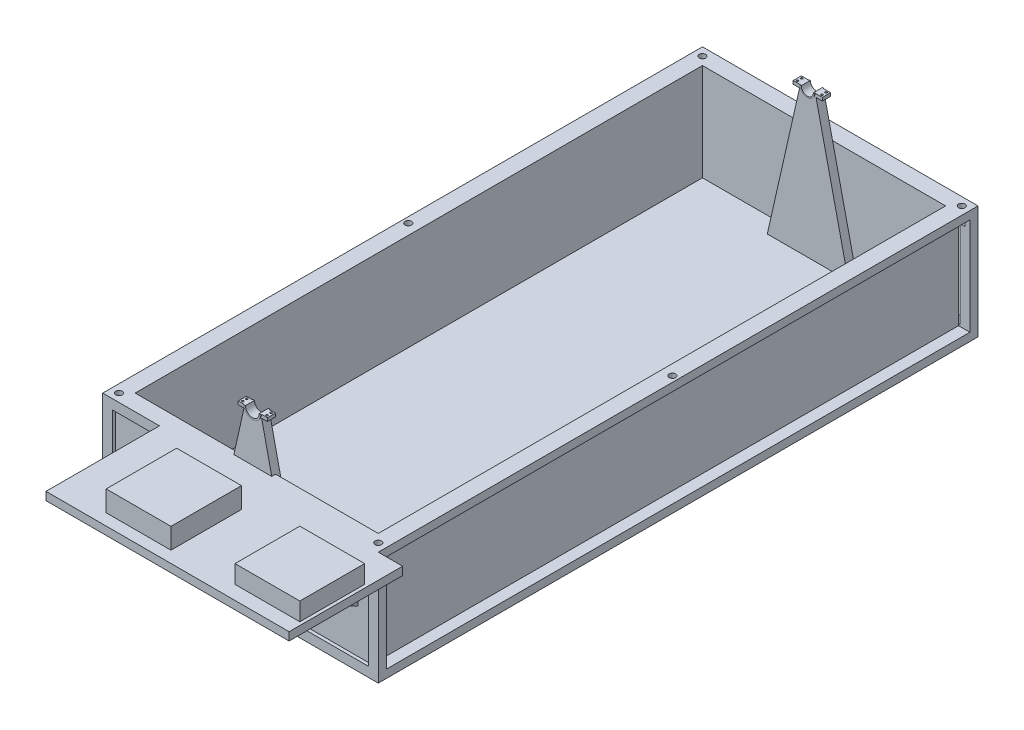
from build123d import *

# Parameters (mm, degrees)
SKETCH_1_R             = 50
SKETCH_1_R_2           = 42.55
EXTRUDE_1_DEPTH        = 50
SKETCH_3_R             = 45
SKETCH_3_R_2           = 37.55
EXTRUDE_2_DEPTH        = 50
EXTRUDE_START          = -50
EXTRUDE_3_DEPTH        = 50
SKETCH_8_R             = 37.55
EXTRUDE_4_DEPTH        = 50
SKETCH_4_W             = 700
SKETCH_4_H             = 3700
EXTRUDE_5_DEPTH        = 100
SKETCH_12_W            = 500
SKETCH_12_H            = 1000
EXTRUDE_6_DEPTH        = 100
SKETCH_16_W            = 500
SKETCH_16_H            = 2700
EXTRUDE_8_DEPTH        = 100
SKETCH_17_W            = 100
SKETCH_17_H            = 100
EXTRUDE_9_DEPTH        = 600
SKETCH_18_W            = 100
SKETCH_18_H            = 100
EXTRUDE_10_DEPTH       = 600
SKETCH_19_W            = 100
SKETCH_19_H            = 100
EXTRUDE_11_DEPTH       = 3500
SKETCH_20_R            = 25
CUT_EXTRUDE_5_DEPTH    = 20
SKETCH_21_R            = 52.5
SKETCH_21_R_2          = 42.55
EXTRUDE_12_DEPTH       = 50
CUT_EXTRUDE_START      = -356
CUT_EXTRUDE_6_DEPTH    = 356
SKETCH_23_W            = 47.45
SKETCH_23_H            = 50
EXTRUDE_13_DEPTH       = 20
CUT_EXTRUDE_8_DEPTH    = 611
SKETCH_26_W            = 52.45
SKETCH_26_H            = 50
EXTRUDE_14_DEPTH       = 20
SKETCH_27_R            = 6
CUT_EXTRUDE_9_DEPTH    = 20
SKETCH_28_R            = 6
CUT_EXTRUDE_10_DEPTH   = 20
EXTRUDE_START_2        = -53
EXTRUDE_15_DEPTH       = 53
EXTRUDE_START_3        = 3
EXTRUDE_16_DEPTH       = 3
EXTRUDE_17_DEPTH       = 3
EXTRUDE_18_DEPTH       = 53
SKETCH_31_W            = 3500
SKETCH_31_H            = 500
EXTRUDE_19_DEPTH       = 100
SKETCH_33_W            = 500
SKETCH_33_H            = 3700
EXTRUDE_20_DEPTH       = 100
EXTRUDE_21_DEPTH       = 100
SKETCH_35_W            = 1500
SKETCH_35_H            = 600
EXTRUDE_22_DEPTH       = 100
SKETCH_36_W            = 1500
SKETCH_36_H            = 600
EXTRUDE_23_DEPTH       = 100
SKETCH_37_W            = 3600
SKETCH_37_H            = 600
CUT_EXTRUDE_11_DEPTH   = 70
SKETCH_38_W            = 1580
SKETCH_38_H            = 580
CUT_EXTRUDE_15_DEPTH   = 50
SKETCH_39_W            = 3600
SKETCH_39_H            = 600
CUT_EXTRUDE_16_DEPTH   = 70
SKETCH_40_W            = 1580
SKETCH_40_H            = 580
CUT_EXTRUDE_17_DEPTH   = 20
SKETCH_43_R            = 20
CUT_EXTRUDE_20_DEPTH   = 100
EXTRUDE_24_DEPTH       = 50
EXTRUDE_25_DEPTH       = 25
PATTERN_LINEAR_1_COUNT = 4
PATTERN_LINEAR_1_PITCH = 100
PATTERN_LINEAR_2_COUNT = 8
PATTERN_LINEAR_2_PITCH = 100
SKETCH_46_W            = 400
SKETCH_46_H            = 435
EXTRUDE_26_DEPTH       = 127.5
SKETCH_47_W            = 400
SKETCH_47_H            = 400
EXTRUDE_28_DEPTH       = 111


with BuildPart() as part:
    # 草图1 → 凸台-拉伸1 (new body)
    with BuildSketch(Plane.XY):
        Circle(SKETCH_1_R)
        Circle(SKETCH_1_R_2, mode=Mode.SUBTRACT)
    extrude(amount=EXTRUDE_1_DEPTH)

    # 草图7 → 凸台-拉伸3 (add)
    with BuildSketch(Plane.XY.offset(50).offset(EXTRUDE_START)):
        with BuildLine():
            ThreePointArc((50, 0), (0, -50), (-50, 0))
            Line((-50, 0), (-250, -900))
            Line((-250, -900), (250, -900))
            Line((250, -900), (50, 0))
        make_face()
    extrude(amount=EXTRUDE_3_DEPTH)



with BuildPart() as body_2:
    # 草图3 → 凸台-拉伸2 (new body)
    with BuildSketch(Plane(origin=(0, 0, -3374), x_dir=(-1, 0, 0), z_dir=(0, 0, -1))):
        Circle(SKETCH_3_R)
        Circle(SKETCH_3_R_2, mode=Mode.SUBTRACT)
    extrude(amount=EXTRUDE_2_DEPTH)

    # 草图8 → 凸台-拉伸4 (add)
    with BuildSketch(Plane(origin=(0, 0, -3424), x_dir=(-1, 0, 0), z_dir=(0, 0, -1))):
        with BuildLine():
            Line((-43.888190419, 9.941164005), (-250, -900))
            Line((-250, -900), (250, -900))
            Line((250, -900), (43.888190419, 9.941164005))
            ThreePointArc((43.888190419, 9.941164005), (0, 45), (-43.888190419, 9.941164005))
        make_face()
        Circle(SKETCH_8_R, mode=Mode.SUBTRACT)
    extrude(amount=-EXTRUDE_4_DEPTH)


with BuildPart() as part_1:
    add(part.part)

    add(body_2.part)  # 凸台-拉伸5 merges body 2
    # 草图4 → 凸台-拉伸5 (add)
    with BuildSketch(Plane(origin=(0, -900, 0), x_dir=(1, 0, 0), z_dir=(0, 1, 0))):
        with Locations((0, 1724)):
            Rectangle(SKETCH_4_W, SKETCH_4_H)
    extrude(amount=-EXTRUDE_5_DEPTH)

    # 草图12 → 凸台-拉伸6 (add)
    with BuildSketch(Plane(origin=(0, -900, 0), x_dir=(1, 0, 0), z_dir=(0, 1, 0))):
        with Locations((600, 374)):
            Rectangle(SKETCH_12_W, SKETCH_12_H)
    extrude(amount=-EXTRUDE_6_DEPTH)

    # 草图16 → 凸台-拉伸8 (add)
    with BuildSketch(Plane(origin=(0, -900, 0), x_dir=(1, 0, 0), z_dir=(0, 1, 0))):
        with Locations((600, 2224)):
            Rectangle(SKETCH_16_W, SKETCH_16_H)
    extrude(amount=-EXTRUDE_8_DEPTH)

    # 草图17 → 凸台-拉伸9 (add)
    with BuildSketch(Plane(origin=(0, -900, 0), x_dir=(1, 0, 0), z_dir=(0, 1, 0))):
        with Locations((800, 3524)):
            Rectangle(SKETCH_17_W, SKETCH_17_H)
    extrude(amount=EXTRUDE_9_DEPTH)

    # 草图18 → 凸台-拉伸10 (add)
    with BuildSketch(Plane(origin=(0, -900, 0), x_dir=(1, 0, 0), z_dir=(0, 1, 0))):
        with Locations((800, -76)):
            Rectangle(SKETCH_18_W, SKETCH_18_H)
    extrude(amount=EXTRUDE_10_DEPTH)

    # 草图19 → 凸台-拉伸11 (add)
    with BuildSketch(Plane.XY.offset(-3474)):
        with Locations((800, -350)):
            Rectangle(SKETCH_19_W, SKETCH_19_H)
    extrude(amount=EXTRUDE_11_DEPTH)

    # 草图20 → 切除-拉伸5 (cut)
    with BuildSketch(Plane.ZY.offset(-750)):
        with Locations((-3424, -350)):
            Circle(SKETCH_20_R)
    extrude(amount=-CUT_EXTRUDE_5_DEPTH, mode=Mode.SUBTRACT)

    # 草图21 → 凸台-拉伸12 (add)
    with BuildSketch(Plane.XY.offset(50).offset(EXTRUDE_START)):
        Circle(SKETCH_21_R)
        Circle(SKETCH_21_R_2, mode=Mode.SUBTRACT)
    extrude(amount=EXTRUDE_12_DEPTH)

    # 草图22 → 切除-拉伸6 (cut)
    with BuildSketch(Plane.XY.offset(50).offset(CUT_EXTRUDE_START)):
        with BuildLine():
            Line((-52.5, 0), (52.5, 0))
            ThreePointArc((52.5, 0), (0, 52.5), (-52.5, 0))
        make_face()
    extrude(amount=CUT_EXTRUDE_6_DEPTH, mode=Mode.SUBTRACT)

    # 草图23 → 凸台-拉伸13 (add)
    with BuildSketch(Plane(origin=(0, 0, 0), x_dir=(1, 0, 0), z_dir=(0, 1, 0))):
        with Locations((-66.275, -25)):
            Rectangle(SKETCH_23_W, SKETCH_23_H)
        with Locations((66.275, -25)):
            Rectangle(SKETCH_23_W, SKETCH_23_H)
    extrude(amount=-EXTRUDE_13_DEPTH)

    # 草图24 → 切除-拉伸8 (cut)
    with BuildSketch(Plane(origin=(0, 0, -3424), x_dir=(-1, 0, 0), z_dir=(0, 0, -1))):
        with BuildLine():
            Line((-55, 0), (55, 0))
            ThreePointArc((55, 0), (0, 55), (-55, 0))
        make_face()
    extrude(amount=-CUT_EXTRUDE_8_DEPTH, mode=Mode.SUBTRACT)

    # 草图26 → 凸台-拉伸14 (add)
    with BuildSketch(Plane(origin=(0, 0, 0), x_dir=(1, 0, 0), z_dir=(0, 1, 0))):
        with Locations((-63.775, 3399)):
            Rectangle(SKETCH_26_W, SKETCH_26_H)
        with Locations((63.775, 3399)):
            Rectangle(SKETCH_26_W, SKETCH_26_H)
    extrude(amount=-EXTRUDE_14_DEPTH)

    # 草图27 → 切除-拉伸9 (cut)
    with BuildSketch(Plane(origin=(0, 0, 0), x_dir=(1, 0, 0), z_dir=(0, 1, 0))):
        with Locations(Location((-75, -12.5, 0), (0, 0, 270))):
            Circle(SKETCH_27_R)
        with Locations(Location((-75, -37.5, 0), (0, 0, 270))):
            Circle(SKETCH_27_R)
        with Locations(Location((75, -37.5, 0), (0, 0, 90))):
            Circle(SKETCH_27_R)
        with Locations(Location((75, -12.5, 0), (0, 0, 90))):
            Circle(SKETCH_27_R)
    extrude(amount=-CUT_EXTRUDE_9_DEPTH, mode=Mode.SUBTRACT)

    # 草图28 → 切除-拉伸10 (cut)
    with BuildSketch(Plane(origin=(0, 0, 0), x_dir=(1, 0, 0), z_dir=(0, 1, 0))):
        with Locations(Location((-75, 3411.5, 0), (0, 0, 270))):
            Circle(SKETCH_28_R)
        with Locations(Location((-75, 3386.5, 0), (0, 0, 270))):
            Circle(SKETCH_28_R)
        with Locations(Location((75, 3386.5, 0), (0, 0, 90))):
            Circle(SKETCH_28_R)
        with Locations(Location((75, 3411.5, 0), (0, 0, 90))):
            Circle(SKETCH_28_R)
    extrude(amount=-CUT_EXTRUDE_10_DEPTH, mode=Mode.SUBTRACT)

    # 草图29 → 凸台-拉伸15 (add)
    with BuildSketch(Plane.XY.offset(50).offset(EXTRUDE_START_2)):
        with BuildLine():
            Line((-52.5, 0), (-42.55, 0))
            ThreePointArc((-42.55, 0), (0, -42.55), (42.55, 0))
            Line((42.55, 0), (52.5, 0))
            ThreePointArc((52.5, 0), (0, -52.5), (-52.5, 0))
        make_face()
    extrude(amount=EXTRUDE_15_DEPTH)

    # 草图30 → 凸台-拉伸16 (add)
    with BuildSketch(Plane.XY.offset(-3374).offset(EXTRUDE_START_3)):
        with BuildLine():
            Line((-45, 0), (-37.55, 0))
            ThreePointArc((-37.55, 0), (0, -37.55), (37.55, 0))
            Line((37.55, 0), (45, 0))
            ThreePointArc((45, 0), (0, -45), (-45, 0))
        make_face()
    extrude(amount=-EXTRUDE_16_DEPTH)

    # 草图29<2> → 凸台-拉伸17 (add)
    with BuildSketch(Plane.XY.offset(50)):
        with BuildLine():
            Line((-52.5, 0), (-42.55, 0))
            ThreePointArc((-42.55, 0), (0, -42.55), (42.55, 0))
            Line((42.55, 0), (52.5, 0))
            ThreePointArc((52.5, 0), (0, -52.5), (-52.5, 0))
        make_face()
    extrude(amount=EXTRUDE_17_DEPTH)

    # 草图30<2> → 凸台-拉伸18 (add)
    with BuildSketch(Plane.XY.offset(-3374)):
        with BuildLine():
            Line((-45, 0), (-37.55, 0))
            ThreePointArc((-37.55, 0), (0, -37.55), (37.55, 0))
            Line((37.55, 0), (45, 0))
            ThreePointArc((45, 0), (0, -45), (-45, 0))
        make_face()
    extrude(amount=-EXTRUDE_18_DEPTH)

    # 草图31 → 凸台-拉伸19 (add)
    with BuildSketch(Plane.ZY.offset(-750)):
        with Locations((-1724, -650)):
            Rectangle(SKETCH_31_W, SKETCH_31_H)
    extrude(amount=-EXTRUDE_19_DEPTH)

    # 草图33 → 凸台-拉伸20 (add)
    with BuildSketch(Plane(origin=(0, -900, 0), x_dir=(1, 0, 0), z_dir=(0, 1, 0))):
        with Locations((-600, 1724)):
            Rectangle(SKETCH_33_W, SKETCH_33_H)
    extrude(amount=-EXTRUDE_20_DEPTH)

    # 草图34 → 凸台-拉伸21 (add)
    with BuildSketch(Plane.ZY.offset(850)):
        Polygon((126, -300), (126, -900), (126, -1000), (-3574, -1000), (-3574, -900), (-3574, -300), align=None)
    extrude(amount=-EXTRUDE_21_DEPTH)

    # 草图35 → 凸台-拉伸22 (add)
    with BuildSketch(Plane(origin=(0, 0, -3574), x_dir=(-1, 0, 0), z_dir=(0, 0, -1))):
        with Locations((0, -600)):
            Rectangle(SKETCH_35_W, SKETCH_35_H)
    extrude(amount=-EXTRUDE_22_DEPTH)

    # 草图36 → 凸台-拉伸23 (add)
    with BuildSketch(Plane.XY.offset(126)):
        with Locations((0, -600)):
            Rectangle(SKETCH_36_W, SKETCH_36_H)
    extrude(amount=-EXTRUDE_23_DEPTH)

    # 草图37 → 切除-拉伸11 (cut)
    with BuildSketch(Plane.ZY.offset(850)):
        with Locations((-1724, -650)):
            Rectangle(SKETCH_37_W, SKETCH_37_H)
    extrude(amount=-CUT_EXTRUDE_11_DEPTH, mode=Mode.SUBTRACT)

    # 草图38 → 切除-拉伸15 (cut)
    with BuildSketch(Plane(origin=(0, 0, -3574), x_dir=(-1, 0, 0), z_dir=(0, 0, -1))):
        with Locations((0, -650)):
            Rectangle(SKETCH_38_W, SKETCH_38_H)
    extrude(amount=-CUT_EXTRUDE_15_DEPTH, mode=Mode.SUBTRACT)

    # 草图39 → 切除-拉伸16 (cut)
    with BuildSketch(Plane(origin=(850, 0, 0), x_dir=(0, 0, -1), z_dir=(1, 0, 0))):
        with Locations((1724, -650)):
            Rectangle(SKETCH_39_W, SKETCH_39_H)
    extrude(amount=-CUT_EXTRUDE_16_DEPTH, mode=Mode.SUBTRACT)

    # 草图40 → 切除-拉伸17 (cut)
    with BuildSketch(Plane.XY.offset(126)):
        with Locations((0, -650)):
            Rectangle(SKETCH_40_W, SKETCH_40_H)
    extrude(amount=-CUT_EXTRUDE_17_DEPTH, mode=Mode.SUBTRACT)

    # 草图43 → 切除-拉伸20 (cut)
    with BuildSketch(Plane(origin=(0, -300, 0), x_dir=(1, 0, 0), z_dir=(0, 1, 0))):
        with Locations(Location((800, 3524, 0), (0, 0, 270))):
            Circle(SKETCH_43_R)
        with Locations(Location((-800, 3524, 0), (0, 0, 270))):
            Circle(SKETCH_43_R)
        with Locations(Location((815, 1724, 0), (0, 0, 270))):
            Circle(SKETCH_43_R)
        with Locations(Location((-815, 1724, 0), (0, 0, 270))):
            Circle(SKETCH_43_R)
        with Locations(Location((800, -76, 0), (0, 0, 180))):
            Circle(SKETCH_43_R)
        with Locations((-800, -76)):
            Circle(SKETCH_43_R)
    extrude(amount=-CUT_EXTRUDE_20_DEPTH, mode=Mode.SUBTRACT)

    # 草图44 → 凸台-拉伸24 (add)
    with BuildSketch(Plane(origin=(0, -300, 0), x_dir=(1, 0, 0), z_dir=(0, 1, 0))):
        Polygon((-500, -126), (-500, -826), (500, -826), (1000, -826), (1000, -126), (500, -126), align=None)
    extrude(amount=-EXTRUDE_24_DEPTH)

    # 草图45 → 凸台-拉伸25 (add, symmetric)
    with BuildSketch(Plane(origin=(0, 0, 0), x_dir=(0, 0, -1), z_dir=(1, 0, 0))):
        Polygon((-726, -350), (-126, -650), (-126, -350), align=None)
    extrude_25 = extrude(amount=EXTRUDE_25_DEPTH, both=True)

    # 阵列(线性)1: 凸台-拉伸25 ×4
    with Locations(*[(-i * PATTERN_LINEAR_1_PITCH, 0, 0) for i in range(1, PATTERN_LINEAR_1_COUNT)]):
        add(extrude_25)

    # 阵列(线性)2: 凸台-拉伸25 ×8
    with Locations(*[(i * PATTERN_LINEAR_2_PITCH, 0, 0) for i in range(1, PATTERN_LINEAR_2_COUNT)]):
        add(extrude_25)

    # 草图46 → 凸台-拉伸26 (add)
    with BuildSketch(Plane(origin=(0, -300, 0), x_dir=(1, 0, 0), z_dir=(0, 1, 0))):
        with Locations((0, -537.5)):
            Rectangle(SKETCH_46_W, SKETCH_46_H)
    extrude(amount=EXTRUDE_26_DEPTH)

    # 草图47 → 凸台-拉伸28 (add)
    with BuildSketch(Plane(origin=(0, -300, 0), x_dir=(1, 0, 0), z_dir=(0, 1, 0))):
        with Locations((780, -540)):
            Rectangle(SKETCH_47_W, SKETCH_47_H)
    extrude(amount=EXTRUDE_28_DEPTH)


solid = part_1.part
